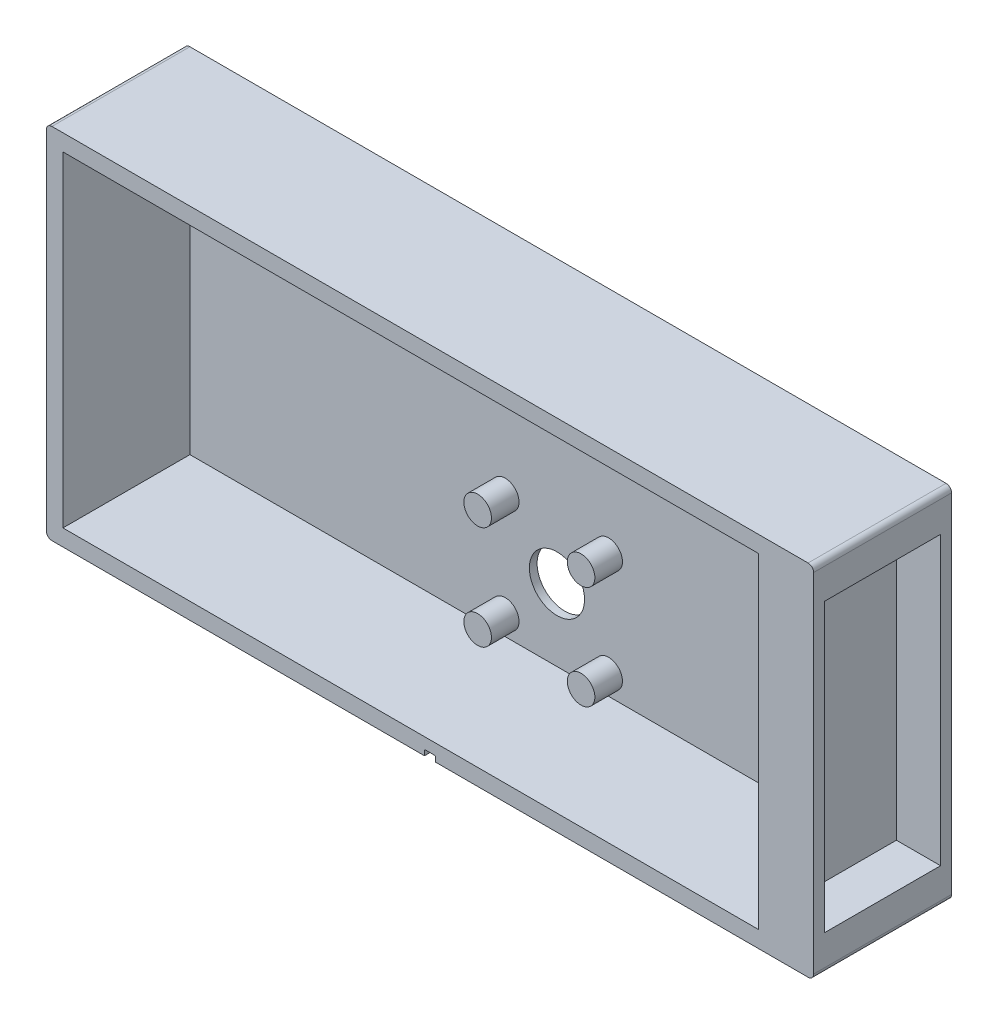
from build123d import *

# Parameters (mm, degrees)
BOSS_EXTRUDE1_DEPTH  = 25
SHELL1_T             = -2
SKETCH6_R            = 10.15
CUT_EXTRUDE3_DEPTH   = 0.6
SKETCH10_R           = 5
CUT_EXTRUDE4_DEPTH   = 81.509999379
SKETCH11_R           = 8
SKETCH11_R_2         = 7
BOSS_EXTRUDE5_DEPTH  = 0.6
SKETCH13_R           = 2.5
BOSS_EXTRUDE6_DEPTH  = 5
CUT_EXTRUDE5_START   = -2
SKETCH15_R           = 0.5
CUT_EXTRUDE5_DEPTH   = 77.806725601
SKETCH16_W           = 2
SKETCH16_H           = 58.164373892
CUT_EXTRUDE6_DEPTH   = 1
FILLET2_R            = 0.1
SKETCH17_R           = 15.5
SKETCH17_R_2         = 10.15
SKETCH17_R_3         = 0.5
BOSS_EXTRUDE7_DEPTH  = 1.2
SKETCH18_W           = 2
SKETCH18_H           = 1.626209188
CUT_EXTRUDE7_DEPTH   = 1
FILLET3_R            = 0.5
FILLET5_R            = 0.2
SKETCH21_W           = 135
SKETCH21_H           = 61
SKETCH21_W_2         = 133
SKETCH21_H_2         = 59
BOSS_EXTRUDE8_DEPTH  = 23
CUT_EXTRUDE8_REACH   = 146.922
SKETCH20_W           = 21
SKETCH20_H           = 52
SKETCH22_W           = 24.612361346
SKETCH22_H           = 60.541750826
SKETCH22_W_2         = 21
SKETCH22_H_2         = 52
BOSS_EXTRUDE9_DEPTH  = 7
SKETCH23_W           = 22.768158453
SKETCH23_H           = 54.342974227
BOSS_EXTRUDE12_DEPTH = 2


with BuildPart() as part:
    # Sketch1 → Boss-Extrude1 (new body)
    with BuildSketch(Plane.XY):
        with BuildLine():
            Line((-68.5, 32.5), (68.5, 32.5))
            ThreePointArc((68.5, 32.5), (69.207106781, 32.207106781), (69.5, 31.5))
            Line((69.5, 31.5), (69.5, -31.5))
            ThreePointArc((69.5, -31.5), (69.207106781, -32.207106781), (68.5, -32.5))
            Line((68.5, -32.5), (-68.5, -32.5))
            ThreePointArc((-68.5, -32.5), (-69.207106781, -32.207106781), (-69.5, -31.5))
            Line((-69.5, -31.5), (-69.5, 31.5))
            ThreePointArc((-69.5, 31.5), (-69.207106781, 32.207106781), (-68.5, 32.5))
        make_face()
    extrude(amount=BOSS_EXTRUDE1_DEPTH)

    # Shell1
    shell1_openings = [part.faces().sort_by_distance(p)[0] for p in [
        (0, 0, 25),
    ]]
    offset(amount=SHELL1_T, openings=shell1_openings, kind=Kind.INTERSECTION)

    # Sketch6 → Cut-Extrude3 (cut)
    with BuildSketch(Plane(origin=(0, 0, 0), x_dir=(-1, 0, 0), z_dir=(0, 0, -1))):
        with Locations((0, -16.5)):
            Circle(SKETCH6_R)
    extrude(amount=-CUT_EXTRUDE3_DEPTH, mode=Mode.SUBTRACT)

    # Sketch10 → Cut-Extrude4 (cut, through all)
    with BuildSketch(Plane(origin=(0, 0, 0.6), x_dir=(-1, 0, 0), z_dir=(0, 0, -1))):
        with Locations((0, -16.5)):
            Circle(SKETCH10_R)
    extrude(amount=-CUT_EXTRUDE4_DEPTH, mode=Mode.SUBTRACT)

    # Sketch11 → Boss-Extrude5 (add)
    with BuildSketch(Plane(origin=(0, 0, 0.6), x_dir=(-1, 0, 0), z_dir=(0, 0, -1))):
        with Locations((0, -16.5)):
            Circle(SKETCH11_R)
        with Locations((0, -16.5)):
            Circle(SKETCH11_R_2, mode=Mode.SUBTRACT)
    extrude(amount=BOSS_EXTRUDE5_DEPTH)

    # Sketch13 → Boss-Extrude6 (add)
    with BuildSketch(Plane.XY.offset(2)):
        with Locations((-9.369164851, -7.130835149)):
            Circle(SKETCH13_R)
        with Locations((9.369164851, -7.130835149)):
            Circle(SKETCH13_R)
        with Locations((9.369164851, -25.869164851)):
            Circle(SKETCH13_R)
        with Locations((-9.369164851, -25.869164851)):
            Circle(SKETCH13_R)
    extrude(amount=BOSS_EXTRUDE6_DEPTH)

    # Sketch15 → Cut-Extrude5 (cut, through all)
    with BuildSketch(Plane.XY.offset(7).offset(CUT_EXTRUDE5_START)):
        with Locations((9.369164851, -7.130835149)):
            Circle(SKETCH15_R)
        with Locations((-9.369164851, -7.130835149)):
            Circle(SKETCH15_R)
        with Locations((-9.369164851, -25.869164851)):
            Circle(SKETCH15_R)
        with Locations((9.369164851, -25.869164851)):
            Circle(SKETCH15_R)
    extrude(amount=-CUT_EXTRUDE5_DEPTH, mode=Mode.SUBTRACT)

    # Sketch16 → Cut-Extrude6 (cut)
    with BuildSketch(Plane(origin=(0, -32.5, 0), x_dir=(-1, 0, 0), z_dir=(0, -1, 0))):
        Rectangle(SKETCH16_W, SKETCH16_H)
    extrude(amount=-CUT_EXTRUDE6_DEPTH, mode=Mode.SUBTRACT)

    # Fillet2
    fillet2_edges = [part.edges().sort_by_distance(p)[0] for p in [
        (7, -16.5, 0.6),
        (8, -16.5, 0),
        (8, -16.5, 0.6),
        (7, -16.5, 0),
    ]]
    fillet(fillet2_edges, radius=FILLET2_R)

    # Sketch17 → Boss-Extrude7 (add)
    with BuildSketch(Plane(origin=(0, 0, 0), x_dir=(-1, 0, 0), z_dir=(0, 0, -1))):
        with Locations(Location((0, -16.5, 0), (0, 0, 266.300928937))):
            Circle(SKETCH17_R)
        with Locations((0, -16.5)):
            Circle(SKETCH17_R_2, mode=Mode.SUBTRACT)
        with Locations(Location((-9.369164851, -7.130835149, 0), (0, 0, 180))):
            Circle(SKETCH17_R_3, mode=Mode.SUBTRACT)
        with Locations(Location((9.369164851, -7.130835149, 0), (0, 0, 180))):
            Circle(SKETCH17_R_3, mode=Mode.SUBTRACT)
        with Locations(Location((9.369164851, -25.869164851, 0), (0, 0, 180))):
            Circle(SKETCH17_R_3, mode=Mode.SUBTRACT)
        with Locations(Location((-9.369164851, -25.869164851, 0), (0, 0, 180))):
            Circle(SKETCH17_R_3, mode=Mode.SUBTRACT)
    extrude(amount=BOSS_EXTRUDE7_DEPTH)

    # Sketch18 → Cut-Extrude7 (cut)
    with BuildSketch(Plane(origin=(0, -32.5, 0), x_dir=(-1, 0, 0), z_dir=(0, -1, 0))):
        with Locations((0, 0.813104594)):
            Rectangle(SKETCH18_W, SKETCH18_H)
    extrude(amount=-CUT_EXTRUDE7_DEPTH, mode=Mode.SUBTRACT)

    # Fillet3
    fillet3_edges = [part.edges().sort_by_distance(p)[0] for p in [
        (2.2125523635452282e-11, -1.0000000000000018, 0),
    ]]
    fillet(fillet3_edges, radius=FILLET3_R)

    # Fillet5
    fillet5_edges = [part.edges().sort_by_distance(p)[0] for p in [
        (1, -31.5, 11.9),
        (-1, -31.5, 11.9),
    ]]
    fillet(fillet5_edges, radius=FILLET5_R)

    # Sketch21 → Boss-Extrude8 (add)
    with BuildSketch(Plane.XY.offset(2)):
        Rectangle(SKETCH21_W, SKETCH21_H)
        Rectangle(SKETCH21_W_2, SKETCH21_H_2, mode=Mode.SUBTRACT)
    extrude(amount=BOSS_EXTRUDE8_DEPTH)

    # Sketch20 → Cut-Extrude8 (cut, up to next)
    with BuildSketch(Plane(origin=(69.5, 0, 0), x_dir=(0, 0, -1), z_dir=(1, 0, 0)), mode=Mode.PRIVATE) as cut_extrude8_sk1:
        with Locations((-12.5, 0)):
            Rectangle(SKETCH20_W, SKETCH20_H)
    cut_extrude8_tool1 = extrude(cut_extrude8_sk1.sketch, amount=-CUT_EXTRUDE8_REACH, mode=Mode.PRIVATE) & part.part
    add(cut_extrude8_tool1.solids().sort_by_distance((69.5, 0, 12.5))[0], mode=Mode.SUBTRACT)

    # Sketch22 → Boss-Extrude9 (add)
    with BuildSketch(Plane.ZY.offset(-66.5)):
        with Locations((12.693819327, -0.195179749)):
            Rectangle(SKETCH22_W, SKETCH22_H)
        with Locations((12.5, 0)):
            Rectangle(SKETCH22_W_2, SKETCH22_H_2, mode=Mode.SUBTRACT)
    extrude(amount=BOSS_EXTRUDE9_DEPTH)

    # Sketch23 → Boss-Extrude12 (add)
    with BuildSketch(Plane.ZY.offset(-59.5)):
        with Locations((12.356599504, -0.189637576)):
            Rectangle(SKETCH23_W, SKETCH23_H)
    extrude(amount=-BOSS_EXTRUDE12_DEPTH)


solid = part.part
